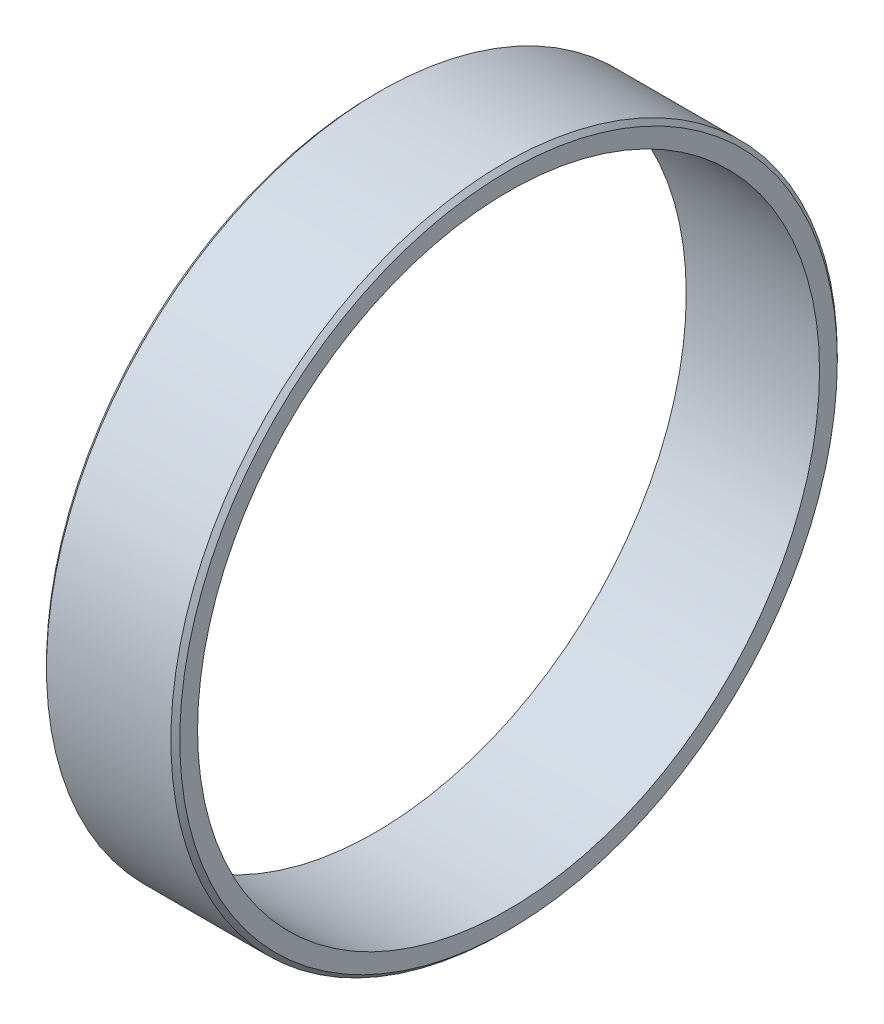
SolidWorks part; units mm, degrees
material "AISI 304"
ref_plane "Front Plane" through (0, 0, 0) normal (0, 0, 1) x (1, 0, 0)
ref_plane "Top Plane" through (0, 0, 0) normal (0, 1, 0) x (1, 0, 0)
ref_plane "Right Plane" through (0, 0, 0) normal (1, 0, 0) x (0, 0, -1)
sketch "Sketch2" plane through (0, 0, 0) normal (1, 0, 0) x (0, 0, -1)
  circle A0 centre (0, 0) radius 35
  circle A1 centre (0, 0) radius 37.5
  dimension "D1" = 70
  dimension "D2" = 75
extrude "Boss-Extrude1" add sketch "Sketch2" against normal blind 15
chamfer "Chamfer1" distance 0.5 angle 45 2 edges at (-15, 0, -37.5) (0, 0, -37.5)
